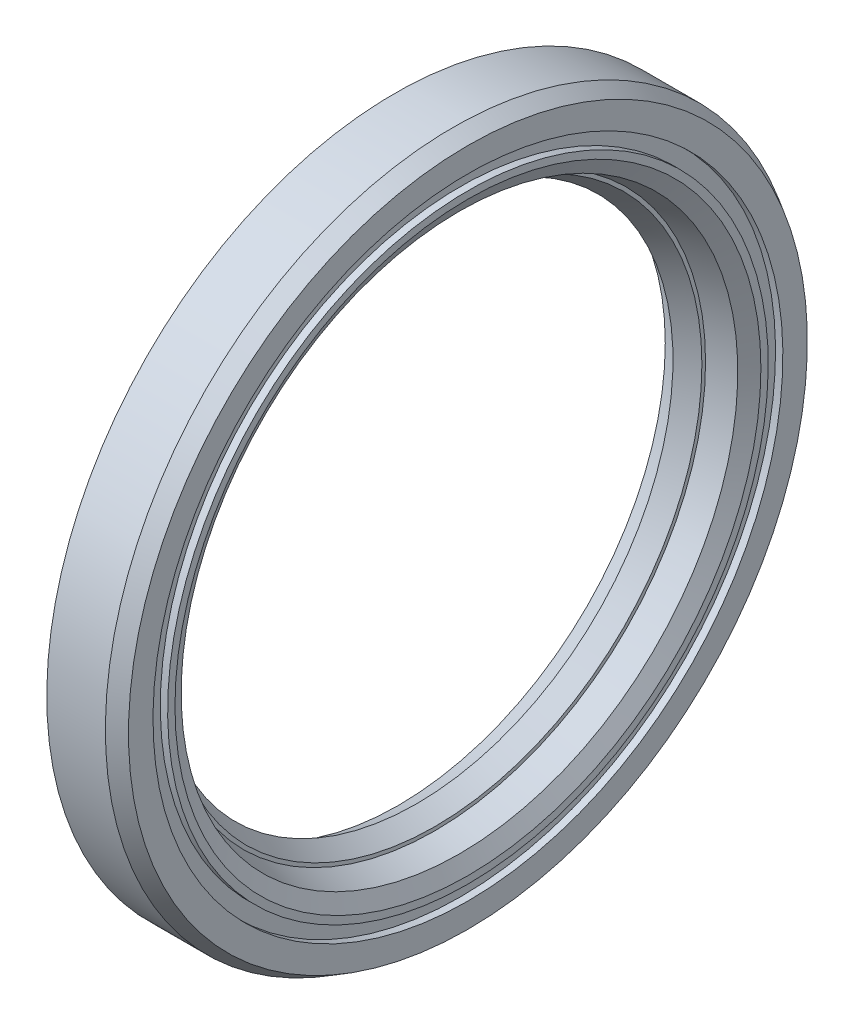
SolidWorks part; units mm, degrees
material "橡胶"
ref_plane "前视基准面" through (0, 0, 0) normal (0, 0, 1) x (1, 0, 0)
ref_plane "上视基准面" through (0, 0, 0) normal (0, 1, 0) x (1, 0, 0)
ref_plane "右视基准面" through (0, 0, 0) normal (1, 0, 0) x (0, 0, -1)
sketch "草图1" plane through (0, 0, 0) normal (0, 0, 1) x (1, 0, 0)
  line L0 (0, 41) -> (0, 40)
  line L1 (0, 0) -> (4.9458, 0) construction
  line L2 (0, 0) -> (0, 40) construction
  line L3 (0, 41) -> (0, 43) construction
  line L4 (-6.9, 39.25) -> (-5.9, 39.25) construction
  line L5 (-9.5, 39.15) -> (-8.7, 39.15) construction
  line L6 (-8.7, 39.15) -> (-7.9, 39.15) construction
  line L7 (-10, 44.5) -> (-10, 0) construction
  line L8 (-3.5, 43.7) -> (-4.3, 43.7) construction
  line L9 (-4.3, 43.7) -> (-4.3, 40.05) construction
  line L10 (-4.3, 40.05) -> (-4.3, 39.25) construction
  line L11 (-3.5, 40.05) -> (-4.3, 40.05) construction
  line L12 (-4.3, 43.7) -> (-4.3, 44.5) construction
  line L13 (-3, 45) -> (-3, 45.5) construction
  line L14 (-3, 45) -> (-2.6464, 45.3536) construction
  line L15 (-3, 45) -> (-2.5, 45) construction
  line L16 (-2, 46.5) -> (-2, 46) construction
  line L17 (-2, 46) -> (-1.5, 46) construction
  line L18 (-2.6464, 45.3536) -> (-2, 46) construction
  line L19 (-2, 46) -> (-1.6464, 46.3536) construction
  line L20 (-6.9, 39.25) -> (-6.9, 39.2) construction
  line L21 (-9.5, 36.4434) -> (-4.5, 36.4434) construction
  line L22 (-7, 36.4434) -> (-7, 35) construction
  line L225 (-10, 44.5) -> (-10, 47.5)
  line L226 (0, 46.3453) -> (0, 43)
  line L230 (-9.5, 39.15) -> (-9.5, 36.4434)
  line L232 (-4.5, 36.9434) -> (-4.5, 36.4434)
  line L233 (-10, 47.5) -> (-2, 47.5)
  line L234 (-2, 47.5) -> (0, 46.3453)
  line L235 (-10, 44.5) -> (-4.3, 44.5)
  line L236 (-3.5, 43.7) -> (-3.5, 40.05)
  line L237 (-4.3, 39.25) -> (-5.9, 39.25)
  line L238 (-9.5, 36.4434) -> (-7, 35)
  line L239 (-7, 35) -> (-4.5, 36.4434)
  line L240 (-4.5, 36.9434) -> (-1.1547, 38)
  line L241 (-1.1547, 38) -> (0, 40)
  line L242 (0, 41) -> (-1, 41)
  line L243 (-1, 41) -> (-1, 43)
  line L244 (-1, 43) -> (0, 43)
  line L245 (-8.5, 46.5) -> (-8.5, 45.5)
  line L246 (-8.5, 46.5) -> (-2, 46.5)
  line L247 (-1.5, 46) -> (-1.5, 41.25)
  line L248 (-1.5, 41.25) -> (-2.5, 41.25)
  line L249 (-2.5, 41.25) -> (-2.5, 45)
  line L250 (-3, 45.5) -> (-8.5, 45.5)
  line L277 (-10, 0) -> (0, 0) construction
  circle A0 centre (-6.9, 39.25) radius 0.8
  circle A1 centre (-6.9, 39.25) radius 0.3
  arc A14 (-7.9, 39.15) -> (-5.9, 39.25) centre (-6.9, 39.2) ccw
  arc A16 (-3.5, 43.7) -> (-4.3, 44.5) centre (-4.3, 43.7) ccw
  arc A17 (-4.3, 39.25) -> (-3.5, 40.05) centre (-4.3, 40.05) ccw
  arc A18 (-7.9, 39.15) -> (-9.5, 39.15) centre (-8.7, 39.15) ccw
  arc A19 (-1.5, 46) -> (-2, 46.5) centre (-2, 46) ccw
  arc A20 (-2.5, 45) -> (-3, 45.5) centre (-3, 45) ccw
  dimension "D1" = 10
  dimension "D9" = 0.8
  dimension "D11" = 0.8
  dimension "D16" = 0.5
  dimension "D23" = 0.5
  dimension "D24" = 1
  dimension "D25" = 0.05
  dimension "D2" = 3
  dimension "D3" = 95
  dimension "D4" = 39.25
  dimension "D5" = 1.5
  dimension "D6" = 1
  dimension "D7" = 1
  dimension "D8" = 70
  dimension "D10" = 0.5
  dimension "D12" = 6.5
  dimension "D13" = 2
  dimension "D14" = 1
  dimension "D15" = 1
  dimension "D17" = 0.5
  dimension "D18" = 4.5
  dimension "D19" = 2
  dimension "D20" = 2
  dimension "D21" = 30
  dimension "D22" = 0.1
  dimension "D26" = 30
  dimension "D27" = 5
  dimension "D28" = 30
  dimension "D29" = 2
  dimension "D30" = 1
  dimension "D31" = 0.5
revolve "旋转1" add sketch "草图1" angle 360 about L277
